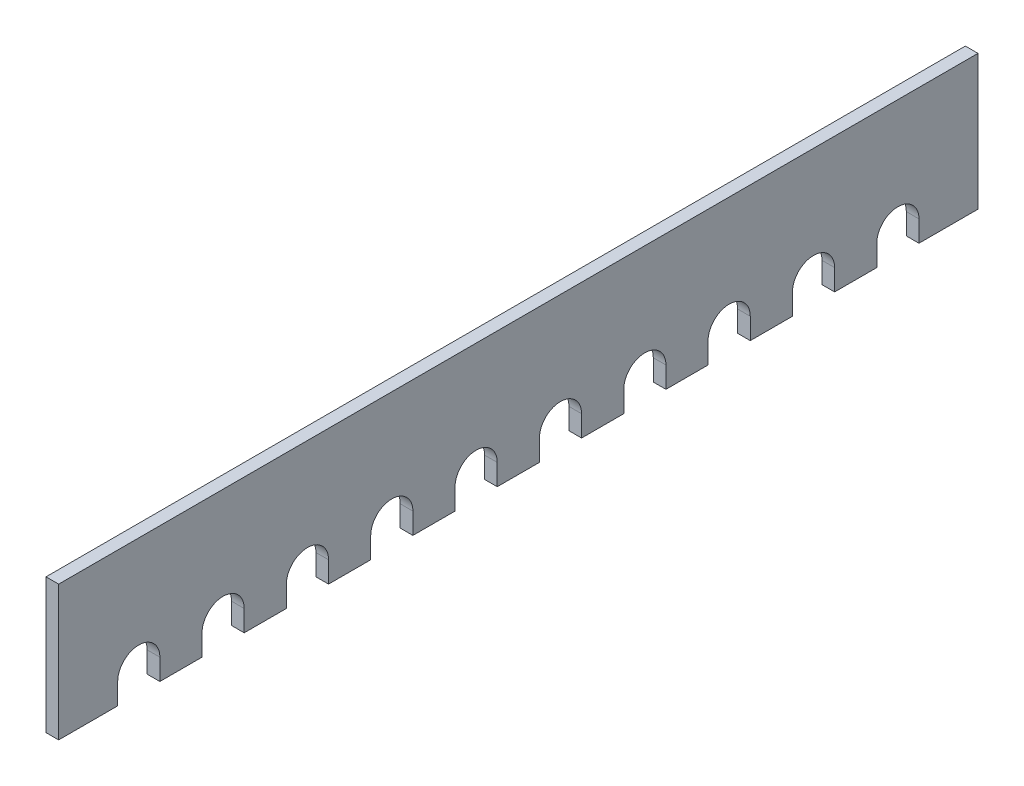
SolidWorks part; units mm, degrees
material "Plain Carbon Steel"
ref_plane "Front Plane" through (0, 0, 0) normal (0, 0, 1) x (1, 0, 0)
ref_plane "Top Plane" through (0, 0, 0) normal (0, 1, 0) x (1, 0, 0)
ref_plane "Right Plane" through (0, 0, 0) normal (1, 0, 0) x (0, 0, -1)
sketch "Sketch1" plane through (0, 0, 0) normal (0, 0, 1) x (1, 0, 0)
  line L1 (0, 0) -> (0, -32)
  dimension "D1" = 32
extrude "Extrude-Thin1" add sketch "Sketch1" along normal blind 218 thin
sketch "Sketch2" plane through (0, 0, 0) normal (1, 0, 0) x (0, 0, -1)
  line L0 (-218, -32) -> (0, -32) construction
  line L1 (-218, 0) -> (-218, -32) construction
  line L2 (-194, -27) -> (-194, -32)
  line L3 (-194, -32) -> (-204, -32)
  line L4 (-204, -32) -> (-204, -27)
  arc A0 (-194, -27) -> (-204, -27) centre (-199, -27) ccw
  dimension "D1" = 10
  dimension "D2" = 5
  dimension "D3" = 19
extrude "Cut-Extrude1" cut sketch "Sketch2" against normal through all
pattern_linear "LPattern1" count 10 spacing 20 along (0, 0, -1) of "Cut-Extrude1"
